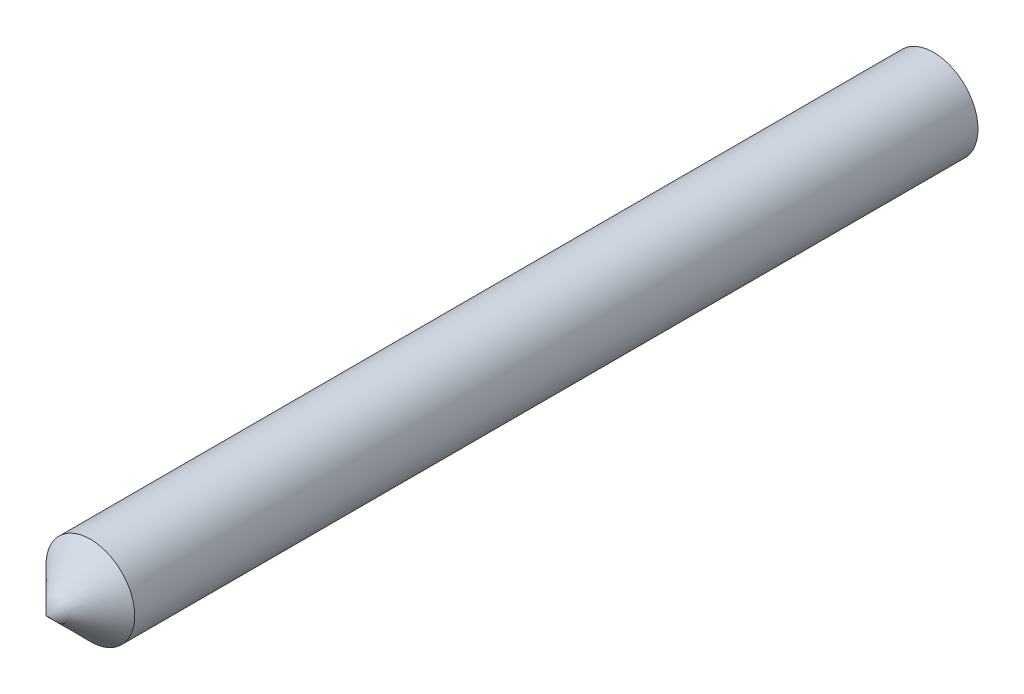
from build123d import *

# Parameters (mm, degrees)
SKETCH1_R           = 5
BOSS_EXTRUDE1_DEPTH = 100
CHAMFER2_SIZE       = 5


with BuildPart() as part:
    # Sketch1 → Boss-Extrude1 (new body)
    with BuildSketch(Plane.XY):
        Circle(SKETCH1_R)
    extrude(amount=BOSS_EXTRUDE1_DEPTH)

    # Chamfer2
    chamfer2_edges = [part.edges().sort_by_distance(p)[0] for p in [
        (-5, 0, 100),
    ]]
    chamfer(chamfer2_edges, length=CHAMFER2_SIZE)


solid = part.part
